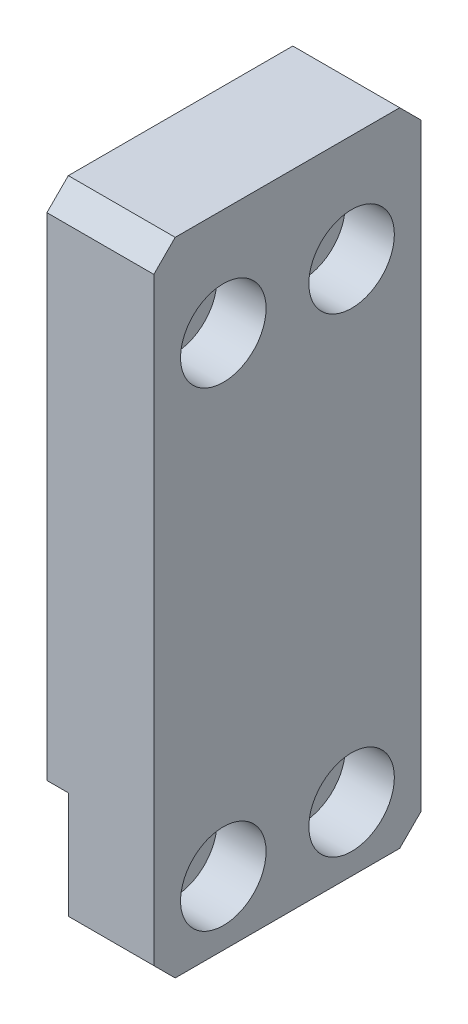
SolidWorks part; units mm, degrees
material "AL6061"
ref_plane "Front Plane" through (0, 0, 0) normal (0, 0, 1) x (1, 0, 0)
ref_plane "Top Plane" through (0, 0, 0) normal (0, 1, 0) x (1, 0, 0)
ref_plane "Right Plane" through (0, 0, 0) normal (1, 0, 0) x (0, 0, -1)
sketch "Sketch1" plane through (0, 0, 0) normal (1, 0, 0) x (0, 0, -1)
  line L1 (-12.5, -30) -> (12.5, -30)
  line L2 (-12.5, -30) -> (-12.5, 30)
  line L3 (-12.5, 30) -> (12.5, 30)
  line L4 (12.5, -30) -> (12.5, 30)
  line L5 (-12.5, -30) -> (12.5, 30) construction
  line L6 (-12.5, 30) -> (12.5, -30) construction
  point P0 (0, 0)
  dimension "D1" = 25
  dimension "D2" = 60
extrude "Boss-Extrude1" add sketch "Sketch1" along normal blind 10
sketch "Sketch4" plane through (0, 0, 0) normal (-1, 0, 0) x (0, 0, 1)
  line L0 (12.5, 30) -> (12.5, -30) construction
  line L1 (-12.5, -30) -> (12.5, -30)
  line L2 (-12.5, -30) -> (-12.5, -18)
  line L3 (-12.5, -18) -> (12.5, -18)
  line L4 (12.5, -30) -> (12.5, -18)
  dimension "D1" = 12
extrude "Cut-Extrude3" cut sketch "Sketch4" against normal blind 2
hole_wizard "CBORE for M4 Hexagon socket head cap screws3" positions "Sketch5" profile "Sketch6" counterbore size "M4" standard "GB" end condition through all
sketch "Sketch5" plane through (10, 0, 0) normal (1, 0, 0) x (0, 0, -1)
  point P0 (-6, -24)
  point P3 (6, -24)
sketch "Sketch6" plane through (10, -24, 6) normal (0, 1, 0) x (0, 0, -1)
  line L0 (0, 0) -> (0, 10)
  line L1 (0, 10) -> (2.25, 10)
  line L3 (2.25, 10) -> (2.25, 4.6)
  line L4 (2.25, 4.6) -> (4, 4.6)
  line L5 (4, 4.6) -> (4, 0)
  line L7 (4, 0) -> (0, 0)
  line L11 (0, -6.35) -> (0, 107.95) construction
  dimension "通孔孔直径" = 4.5
  dimension "通孔孔深度" = 10
  dimension "柱形沉头孔直径" = 8
  dimension "柱形沉头孔深度" = 4.6
hole_wizard "CBORE for M4 Hexagon socket head cap screws4" positions "Sketch7" profile "Sketch8" counterbore size "M4" standard "GB" end condition through all
sketch "Sketch7" plane through (10, 0, 0) normal (1, 0, 0) x (0, 0, -1)
  line L0 (0, 30) -> (0, -30) construction
  line L1 (12.5, 30) -> (-12.5, 30) construction
  line L2 (-12.5, -30) -> (12.5, -30) construction
  point P9 (-6, 20)
  point P11 (6, 20)
  dimension "D1" = 12
  dimension "D2" = 10
sketch "Sketch8" plane through (10, 20, -6) normal (0, 1, 0) x (0, 0, -1)
  line L0 (0, 0) -> (0, 10)
  line L1 (0, 10) -> (2.25, 10)
  line L3 (2.25, 10) -> (2.25, 4.6)
  line L4 (2.25, 4.6) -> (4, 4.6)
  line L5 (4, 4.6) -> (4, 0)
  line L7 (4, 0) -> (0, 0)
  line L11 (0, -6.35) -> (0, 107.95) construction
  dimension "通孔孔直径" = 4.5
  dimension "通孔孔深度" = 10
  dimension "柱形沉头孔直径" = 8
  dimension "柱形沉头孔深度" = 4.6
chamfer "Chamfer1" distance 2 angle 45 4 edges at (5, 30, 12.5) (5, 30, -12.5) (6, -30, 12.5) (6, -30, -12.5)
